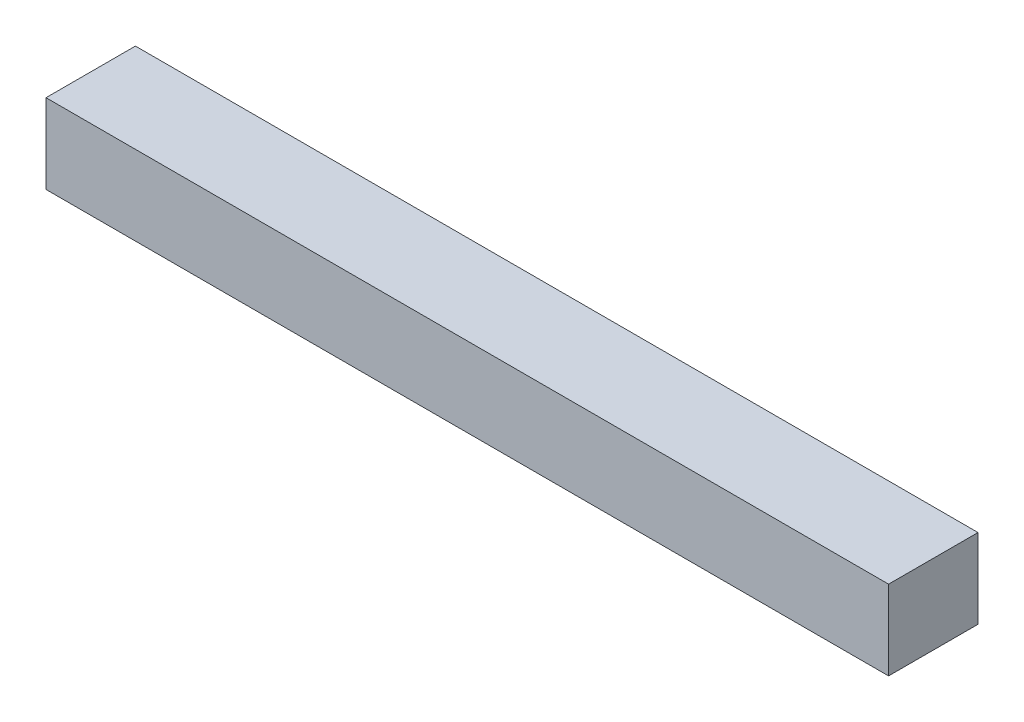
SolidWorks part; units mm, degrees
ref_plane "前视基准面" through (0, 0, 0) normal (0, 0, 1) x (1, 0, 0)
ref_plane "上视基准面" through (0, 0, 0) normal (0, 1, 0) x (1, 0, 0)
ref_plane "右视基准面" through (0, 0, 0) normal (1, 0, 0) x (0, 0, -1)
sketch "草图1" plane through (0, 0, 0) normal (0, 0, 1) x (1, 0, 0)
  line L1 (-2120, 200) -> (2120, 200)
  line L2 (-2120, 200) -> (-2120, -200)
  line L3 (-2120, -200) -> (2120, -200)
  line L4 (2120, 200) -> (2120, -200)
  line L5 (-2120, 200) -> (2120, -200) construction
  line L6 (-2120, -200) -> (2120, 200) construction
  point P0 (0, 0)
  dimension "D1" = 4240
  dimension "D2" = 400
extrude "凸台-拉伸1" add sketch "草图1" along normal blind 450
